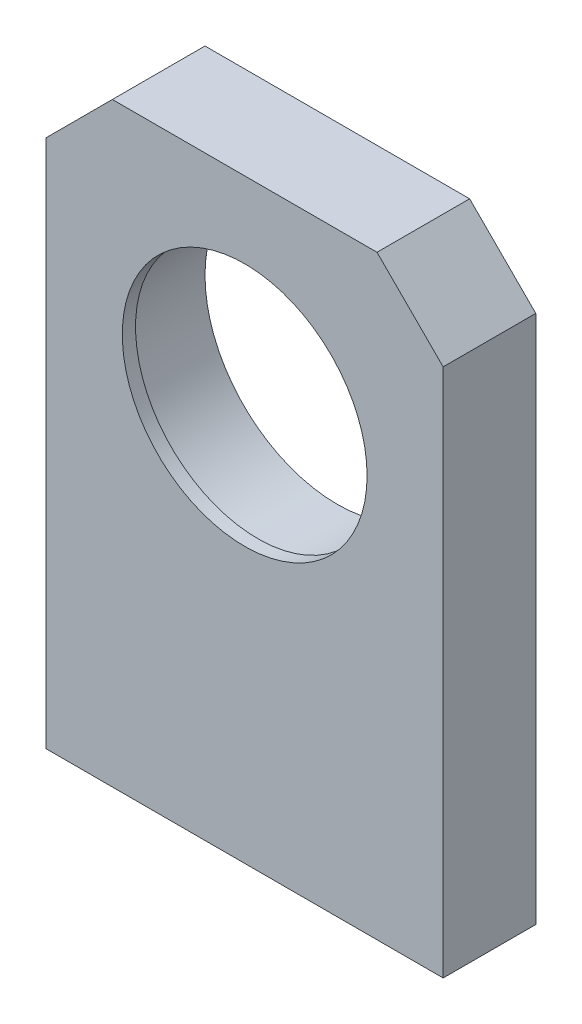
from build123d import *

# Parameters (mm, degrees)
SKETCH_1_W             = 60
SKETCH_1_H             = 90
SKETCH_1_R             = 20
EXTRUDE_1_DEPTH        = 7
EXTRUDE_START          = -2
SKETCH_2_R             = 20
SKETCH_2_R_2           = 18.5
EXTRUDE_2_DEPTH        = 2
CHAMFER_1_SIZE         = 10
HOLE_WIZARD_M6_1_D     = 5
HOLE_WIZARD_M6_1_DEPTH = 14
HOLE_WIZARD_M6_1_TIP   = 1.502151548


with BuildPart() as part:
    # 草图1 → 凸台-拉伸1 (new, symmetric)
    with BuildSketch(Plane.XY):
        Rectangle(SKETCH_1_W, SKETCH_1_H)
        with Locations((0, 15)):
            Circle(SKETCH_1_R, mode=Mode.SUBTRACT)
    extrude(amount=EXTRUDE_1_DEPTH, both=True)

    # 草图2 → 凸台-拉伸2 (add)
    with BuildSketch(Plane.XY.offset(7).offset(EXTRUDE_START)):
        with Locations((0, 15)):
            Circle(SKETCH_2_R)
        with Locations((0, 15)):
            Circle(SKETCH_2_R_2, mode=Mode.SUBTRACT)
    extrude(amount=EXTRUDE_2_DEPTH)

    # 倒角1
    chamfer_1_edges = [part.edges().sort_by_distance(p)[0] for p in [
        (-30, 45, 0),
        (30, 45, 0),
    ]]
    chamfer(chamfer_1_edges, length=CHAMFER_1_SIZE)

    # M6 螺纹孔1
    with Locations(Plane(origin=(-24, -45, 0), x_dir=(0, 0, -1), z_dir=(0, -1, 0))):
        with Locations((0, 0), (0, 48)):
            Hole(HOLE_WIZARD_M6_1_D / 2, depth=HOLE_WIZARD_M6_1_DEPTH)
            with Locations((0, 0, -(HOLE_WIZARD_M6_1_DEPTH + HOLE_WIZARD_M6_1_TIP / 2))):  # 118° drill point
                Cone(0, HOLE_WIZARD_M6_1_D / 2, HOLE_WIZARD_M6_1_TIP, mode=Mode.SUBTRACT)


solid = part.part
